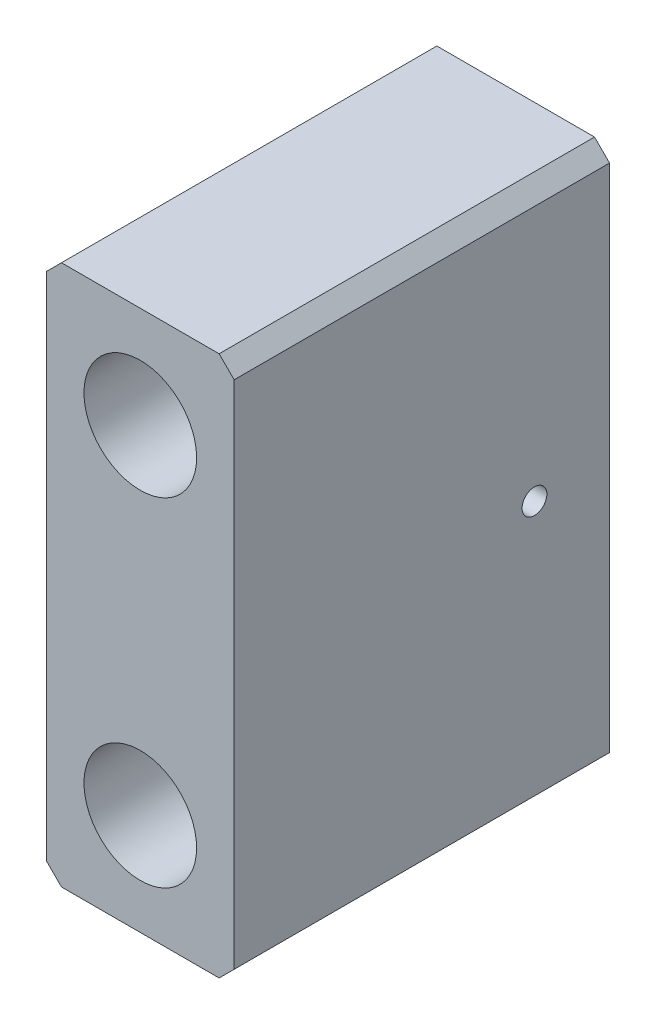
SolidWorks part; units mm, degrees
ref_plane "前视基准面" through (0, 0, 0) normal (0, 0, 1) x (1, 0, 0)
ref_plane "上视基准面" through (0, 0, 0) normal (0, 1, 0) x (1, 0, 0)
ref_plane "右视基准面" through (0, 0, 0) normal (1, 0, 0) x (0, 0, -1)
sketch "草图1" plane through (0, 0, 0) normal (0, 0, 1) x (1, 0, 0)
  line L1 (-12.5, -36) -> (12.5, -36)
  line L2 (-12.5, -36) -> (-12.5, 36)
  line L3 (-12.5, 36) -> (12.5, 36)
  line L4 (12.5, -36) -> (12.5, 36)
  line L5 (-12.5, -36) -> (12.5, 36) construction
  line L6 (-12.5, 36) -> (12.5, -36) construction
  circle A0 centre (0, 22.5) radius 7.5
  circle A1 centre (0, -22.5) radius 7.5
  point P0 (0, 0)
  point P10 (19.9974, 43.9941)
  point P11 (0, 0)
  point P12 (15.0047, 35.4771)
extrude "凸台-拉伸1" add sketch "草图1" along normal blind 50
hole_wizard "M4 螺纹孔1" positions "3D草图1" profile "草图2" tap size "M4" standard "GB"
sketch3d "3D草图1"
  line L0 (12.5, 0, 0) -> (12.5, 0, 10)
  line L1 (12.5, -36, 0) -> (12.5, 36, 0) construction
  point P0 (12.5, 0, 10)
  dimension "D1" = 10
sketch "草图2" plane through (12.5, 0, 10) normal (0, 1, 0) x (0, 0, -1)
  line L0 (0, 0) -> (0, 9.0914)
  line L1 (0, 9.0914) -> (1.65, 8.1)
  line L2 (1.65, 8.1) -> (1.65, 0)
  line L5 (1.65, 0) -> (0, 0)
  line L10 (0, 9.0914) -> (-1.65, 8.1) construction
  line L11 (0, -6.35) -> (0, 107.95) construction
  dimension "螺纹孔钻头直径" = 3.3
  dimension "螺纹孔钻头深度" = 8.1
  dimension "导头角度" = 118
cosmetic thread "孔螺蚊线1"
chamfer "倒角1" distance 2 angle 45 4 edges at (-12.5, -36, 25) (12.5, -36, 25) (-12.5, 36, 25) (12.5, 36, 25)
equation "\"D2@草图1\"=\"D1@草图1\""
